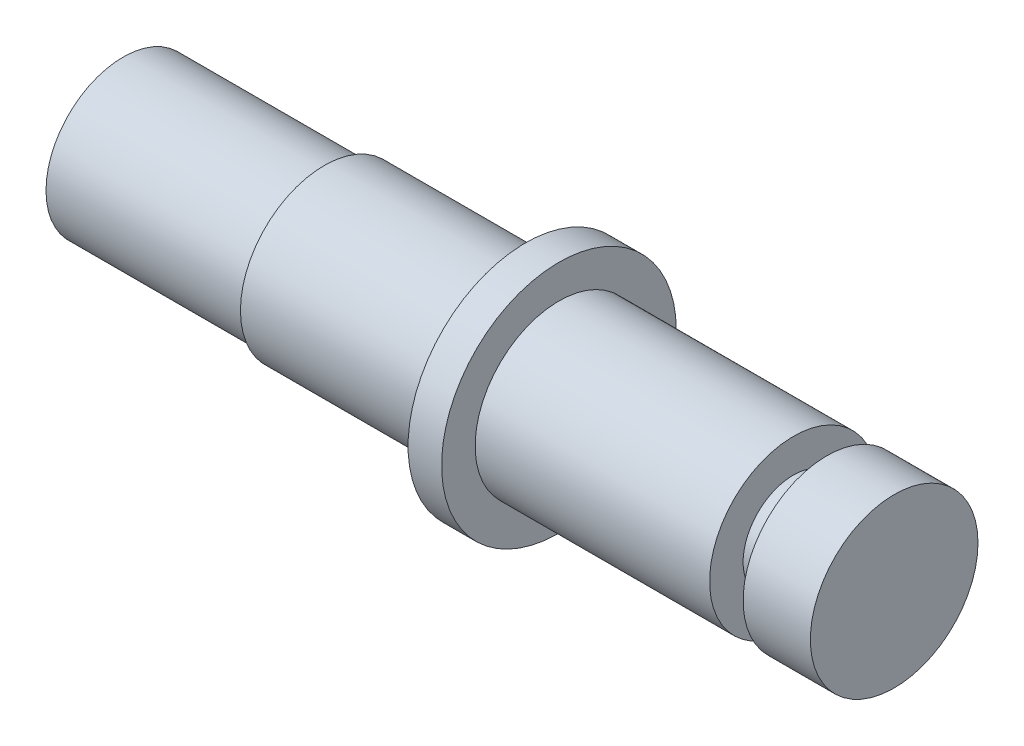
from build123d import *

# Parameters (mm, degrees)
SKETCH1_R           = 2.3
BOSS_EXTRUDE1_DEPTH = 20
SKETCH3_W           = 0.694541754
SKETCH3_H           = 0.2
BOSS_EXTRUDE2_START = 2
SKETCH4_R           = 2.3
BOSS_EXTRUDE2_DEPTH = 2
SKETCH5_R           = 2.5
BOSS_EXTRUDE3_DEPTH = 10
SKETCH6_W           = 1
SKETCH6_H           = 1.000091558
SKETCH10_R          = 2.5
BOSS_EXTRUDE4_DEPTH = 6
SKETCH11_W          = 1
SKETCH11_H          = 1
BOSS_EXTRUDE5_START = 1
SKETCH12_R          = 2.5
BOSS_EXTRUDE5_DEPTH = 1


with BuildPart() as part:
    # Sketch1 → Boss-Extrude1 (new body)
    with BuildSketch(Plane(origin=(0, 0, 0), x_dir=(0, 0, -1), z_dir=(1, 0, 0))):
        Circle(SKETCH1_R)
    extrude(amount=BOSS_EXTRUDE1_DEPTH)

    # Sketch3 → Revolve1 (revolve)
    with BuildSketch(Plane.XY, mode=Mode.PRIVATE) as revolve1_sk:
        with Locations((10.347270877, 2.4)):
            Rectangle(SKETCH3_W, SKETCH3_H)
    revolve(revolve1_sk.sketch.rotate(Axis((20, 0, 0), (-1, 0, 0)), 270), axis=Axis((20, 0, 0), (-1, 0, 0)))

    # Sketch4 → Boss-Extrude2 (add)
    with BuildSketch(Plane.ZY.offset(BOSS_EXTRUDE2_START)):
        Circle(SKETCH4_R)
    extrude(amount=-BOSS_EXTRUDE2_DEPTH)

    # Sketch5 → Boss-Extrude3 (add)
    with BuildSketch(Plane(origin=(20, 0, 0), x_dir=(0, 0, -1), z_dir=(1, 0, 0))):
        with Locations(Location((0, 0, 0), (0, 0, 180))):
            Circle(SKETCH5_R)
    extrude(amount=-BOSS_EXTRUDE3_DEPTH)

    # Sketch6 → Cut-Revolve1 (revolve, cut)
    with BuildSketch(Plane(origin=(0.993947206, 0, 0), x_dir=(1, 0, 0), z_dir=(0, 0, 1)), mode=Mode.PRIVATE) as cut_revolve1_sk:
        with Locations((17.5, 1.999954221)):
            Rectangle(SKETCH6_W, SKETCH6_H)
    revolve(cut_revolve1_sk.sketch.rotate(Axis((20.993947206, 0, 0), (-1, 0, 0)), 270), axis=Axis((20.993947206, 0, 0), (-1, 0, 0)), mode=Mode.SUBTRACT)

    # Sketch10 → Boss-Extrude4 (add)
    with BuildSketch(Plane.ZY.offset(-10)):
        Circle(SKETCH10_R)
    extrude(amount=BOSS_EXTRUDE4_DEPTH)

    # Sketch11 → Revolve2 (revolve)
    with BuildSketch(Plane.XY, mode=Mode.PRIVATE) as revolve2_sk:
        with Locations((10.5, 3)):
            Rectangle(SKETCH11_W, SKETCH11_H)
    revolve(revolve2_sk.sketch.rotate(Axis((20, 0, 0), (-1, 0, 0)), 90), axis=Axis((20, 0, 0), (-1, 0, 0)))

    # Sketch12 → Boss-Extrude5 (add)
    with BuildSketch(Plane(origin=(20, 0, 0), x_dir=(0, 0, -1), z_dir=(1, 0, 0)).offset(BOSS_EXTRUDE5_START)):
        Circle(SKETCH12_R)
    extrude(amount=-BOSS_EXTRUDE5_DEPTH)


solid = part.part
